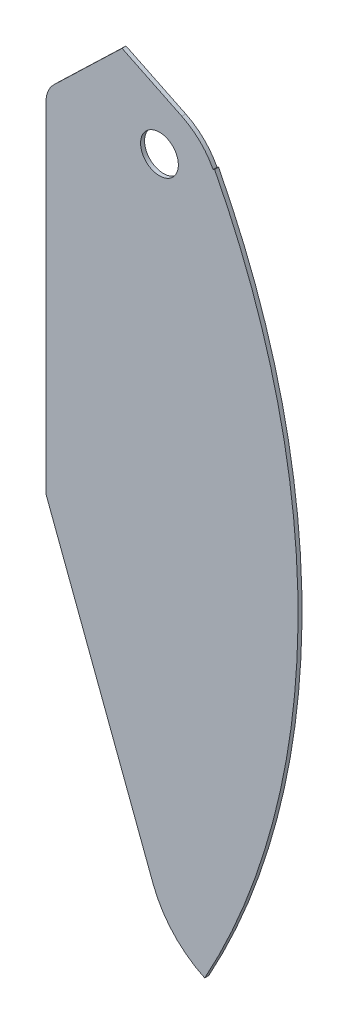
SolidWorks part; units mm, degrees
material "普通碳钢"
ref_plane "Front Plane" through (0, 0, 0) normal (0, 0, 1) x (1, 0, 0)
ref_plane "Top Plane" through (0, 0, 0) normal (0, 1, 0) x (1, 0, 0)
ref_plane "Right Plane" through (0, 0, 0) normal (1, 0, 0) x (0, 0, -1)
sketch "Sketch1" plane through (0, 0, 0) normal (0, 0, 1) x (1, 0, 0)
  line L0 (0, 0) -> (1508.125, 0) construction
  line L1 (1508.125, 1852.0089) -> (1508.125, -1551.2193) construction
  line L2 (1000.125, 641.35) -> (1000.125, -45.0629)
  line L3 (1153.3187, 810.4187) -> (1941.9803, 810.4187) construction
  line L4 (-193.0615, -729.4563) -> (2125.7144, -729.4563) construction
  line L5 (895.3353, 641.35) -> (1099.6798, 641.35) construction
  line L6 (1050.925, 699.3213) -> (1050.925, 510.7757) construction
  line L7 (1153.3187, 810.4187) -> (1015.6958, 677.9498)
  line L8 (1000.125, -45.0629) -> (1215.9344, -617.1138)
  line L9 (1015.6958, 677.9498) -> (1000.125, 662.9621) construction
  line L10 (1153.3187, 810.4187) -> (1273.8245, 751.9596)
  line L11 (1339.9139, 692.15) -> (1336.8708, 690.5722)
  line L12 (1000.125, 641.35) -> (1000.125, 662.9621) construction
  arc A0 (1319.9752, -729.4563) -> (1339.9139, 692.15) centre (0, 0) ccw
  arc A1 (1015.6958, 677.9498) -> (1000.125, 641.35) centre (1050.925, 641.35) ccw
  circle A2 centre (1319.9752, -729.4563) radius 203.2 construction
  arc A3 (1215.9344, -617.1138) -> (1319.9752, -729.4563) centre (1406.0551, -545.3897) ccw
  arc A4 (1336.8708, 690.5722) -> (1273.8245, 751.9596) centre (1212.85, 626.2687) ccw
  circle A5 centre (1228.725, 663.575) radius 38.1
  dimension "D2" = 508
  dimension "D7" = 101.6
  dimension "D9" = 708.025
  dimension "D10" = 406.4
  dimension "D11" = 626.2687
  dimension "D13" = 279.4
  dimension "D15" = 279.4
  dimension "D17" = 76.2
  dimension "D1" = 1508.125
  dimension "D3" = 810.4187
  dimension "D4" = 1539.875
  dimension "D6" = 169.0687
  dimension "D8" = 354.8062
  dimension "D12" = 295.275
  dimension "D14" = 692.15
  dimension "D16" = 663.575
extrude "Boss-Extrude1" add sketch "Sketch1" along normal mid plane 8
